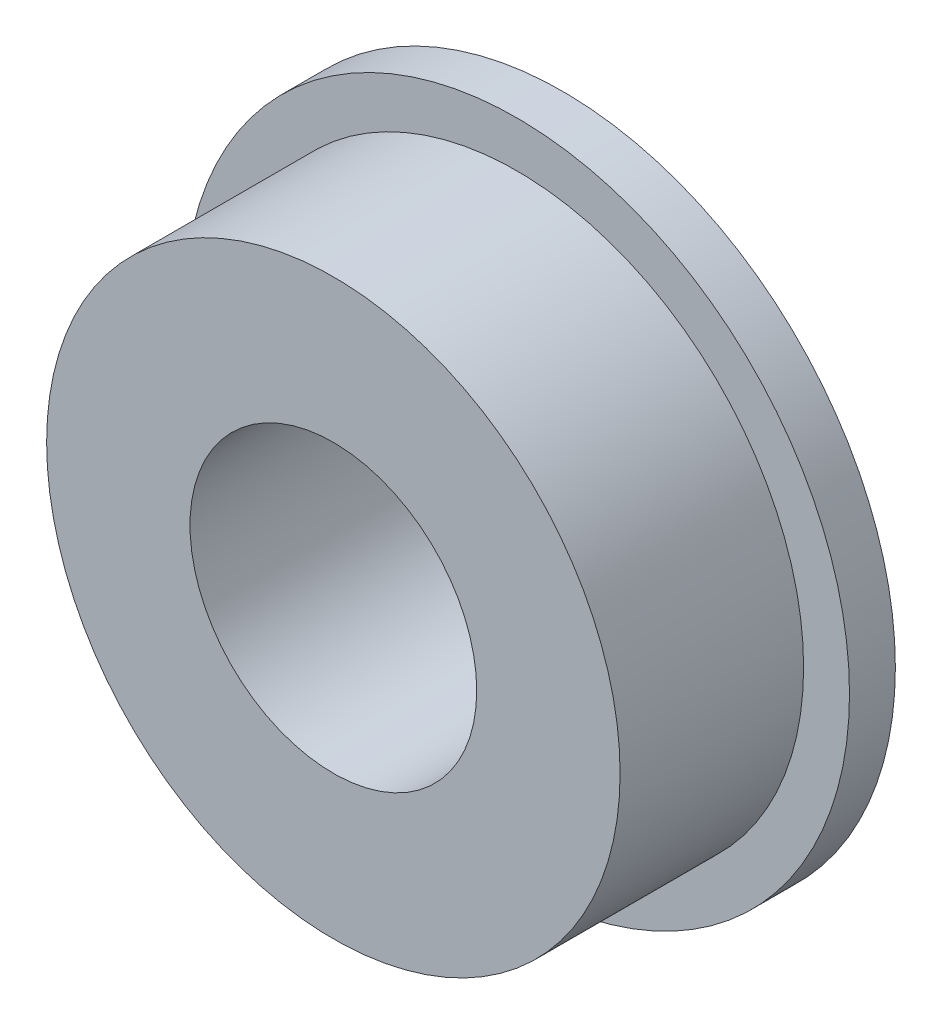
from build123d import *

# Parameters (mm, degrees)
SKETCH_1_R      = 5.8
SKETCH_1_R_2    = 2.5
EXTRUDE_1_DEPTH = 0.8
SKETCH_2_R      = 5
SKETCH_2_R_2    = 2.5
EXTRUDE_2_DEPTH = 3.2


with BuildPart() as part:
    # 草图1 → 凸台-拉伸1 (new body)
    with BuildSketch(Plane.XY):
        Circle(SKETCH_1_R)
        Circle(SKETCH_1_R_2, mode=Mode.SUBTRACT)
    extrude(amount=EXTRUDE_1_DEPTH)

    # 草图2 → 凸台-拉伸2 (add)
    with BuildSketch(Plane.XY.offset(0.8)):
        Circle(SKETCH_2_R)
        Circle(SKETCH_2_R_2, mode=Mode.SUBTRACT)
    extrude(amount=EXTRUDE_2_DEPTH)


solid = part.part
